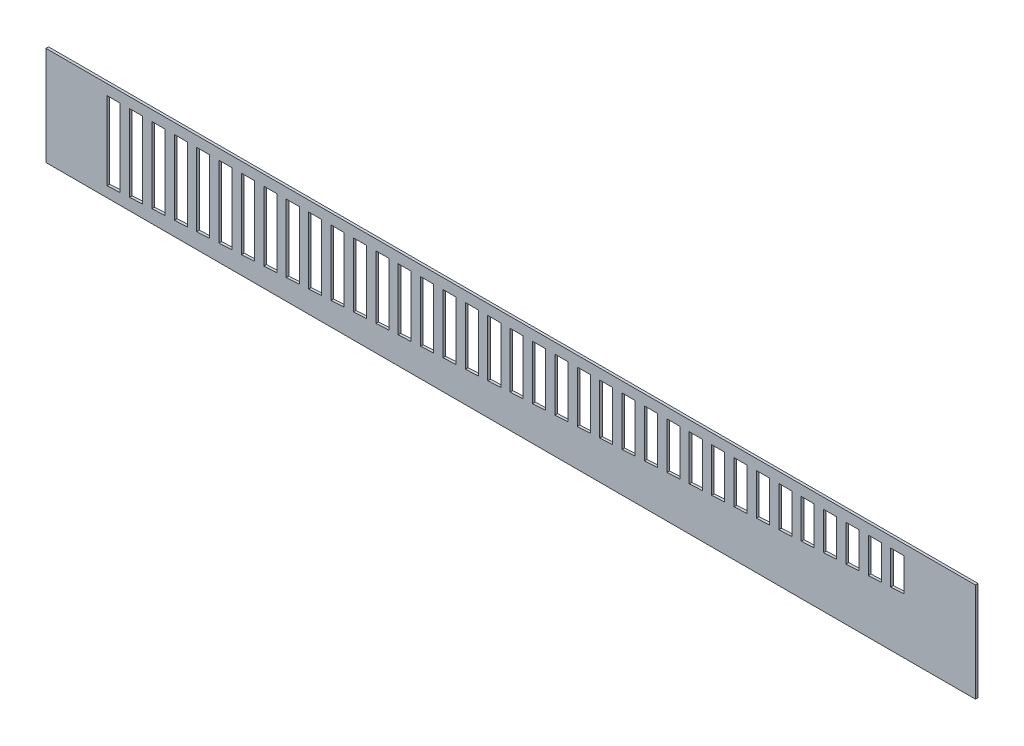
from build123d import *

# Parameters (mm, degrees)
SKETCH1_W           = 178.5
SKETCH1_H           = 19
BOSS_EXTRUDE1_DEPTH = 0.5
CUT_EXTRUDE1_DEPTH  = 147.56


with BuildPart() as part:
    # Sketch1 → Boss-Extrude1 (new body)
    with BuildSketch(Plane.XY):
        Rectangle(SKETCH1_W, SKETCH1_H)
    extrude(amount=BOSS_EXTRUDE1_DEPTH)

    # Sketch2 → Cut-Extrude1 (cut)
    with BuildSketch(Plane.XY.offset(0.5)):
        Polygon((-77.51, 7.5), (-75.01, 7.5), (-75.01, -7.358477447), (-77.51, -7.5), align=None)
        Polygon((-70.71, 7.5), (-70.71, -7.115058656), (-73.21, -7.256581209), (-73.21, 7.5), align=None)
        Polygon((-66.41, 7.5), (-66.41, -6.871639865), (-68.91, -7.013162418), (-68.91, 7.5), align=None)
        Polygon((-62.11, 7.5), (-62.11, -6.628221074), (-64.61, -6.769743627), (-64.61, 7.5), align=None)
        Polygon((-57.81, 7.5), (-57.81, -6.384802283), (-60.31, -6.526324836), (-60.31, 7.5), align=None)
        Polygon((-53.51, 7.5), (-53.51, -6.141383492), (-56.01, -6.282906045), (-56.01, 7.5), align=None)
        Polygon((-49.21, 7.5), (-49.21, -5.897964701), (-51.71, -6.039487254), (-51.71, 7.5), align=None)
        Polygon((-44.91, 7.5), (-44.91, -5.65454591), (-47.41, -5.796068463), (-47.41, 7.5), align=None)
        Polygon((-40.61, 7.5), (-40.61, -5.411127119), (-43.11, -5.552649672), (-43.11, 7.5), align=None)
        Polygon((-36.31, 7.5), (-36.31, -5.167708328), (-38.81, -5.309230881), (-38.81, 7.5), align=None)
        Polygon((-32.01, 7.5), (-32.01, -4.924289537), (-34.51, -5.06581209), (-34.51, 7.5), align=None)
        Polygon((-27.71, 7.5), (-27.71, -4.680870746), (-30.21, -4.822393299), (-30.21, 7.5), align=None)
        Polygon((-23.41, 7.5), (-23.41, -4.437451955), (-25.91, -4.578974508), (-25.91, 7.5), align=None)
        Polygon((-19.11, 7.5), (-19.11, -4.194033164), (-21.61, -4.335555717), (-21.61, 7.5), align=None)
        Polygon((-14.81, 7.5), (-14.81, -3.950614373), (-17.31, -4.092136926), (-17.31, 7.5), align=None)
        Polygon((-10.51, 7.5), (-10.51, -3.707195582), (-13.01, -3.848718135), (-13.01, 7.5), align=None)
        Polygon((-6.21, 7.5), (-6.21, -3.463776791), (-8.71, -3.605299344), (-8.71, 7.5), align=None)
        Polygon((-1.91, 7.5), (-1.91, -3.220358), (-4.41, -3.361880553), (-4.41, 7.5), align=None)
        Polygon((2.39, 7.5), (2.39, -2.976939209), (-0.11, -3.118461762), (-0.11, 7.5), align=None)
        Polygon((6.69, 7.5), (6.69, -2.733520418), (4.19, -2.875042971), (4.19, 7.5), align=None)
        Polygon((10.99, 7.5), (10.99, -2.490101627), (8.49, -2.63162418), (8.49, 7.5), align=None)
        Polygon((15.29, 7.5), (15.29, -2.246682836), (12.79, -2.388205389), (12.79, 7.5), align=None)
        Polygon((19.59, 7.5), (19.59, -2.003264045), (17.09, -2.144786598), (17.09, 7.5), align=None)
        Polygon((23.89, 7.5), (23.89, -1.759845254), (21.39, -1.901367807), (21.39, 7.5), align=None)
        Polygon((28.19, 7.5), (28.19, -1.516426463), (25.69, -1.657949016), (25.69, 7.5), align=None)
        Polygon((32.49, 7.5), (32.49, -1.273007672), (29.99, -1.414530225), (29.99, 7.5), align=None)
        Polygon((36.79, 7.5), (36.79, -1.029588881), (34.29, -1.171111434), (34.29, 7.5), align=None)
        Polygon((41.09, 7.5), (41.09, -0.78617009), (38.59, -0.927692643), (38.59, 7.5), align=None)
        Polygon((45.39, 7.5), (45.39, -0.542751299), (42.89, -0.684273852), (42.89, 7.5), align=None)
        Polygon((49.69, 7.5), (49.69, -0.299332508), (47.19, -0.440855061), (47.19, 7.5), align=None)
        Polygon((53.99, 7.5), (53.99, -0.055913717), (51.49, -0.19743627), (51.49, 7.5), align=None)
        Polygon((58.29, 7.5), (58.29, 0.187505074), (55.79, 0.045982521), (55.79, 7.5), align=None)
        Polygon((62.59, 7.5), (62.59, 0.430923865), (60.09, 0.289401312), (60.09, 7.5), align=None)
        Polygon((66.89, 7.5), (66.89, 0.674342656), (64.39, 0.532820103), (64.39, 7.5), align=None)
        Polygon((71.19, 7.5), (71.19, 0.917761447), (68.69, 0.776238894), (68.69, 7.5), align=None)
        Polygon((75.49, 7.5), (75.49, 1.161180238), (72.99, 1.019657685), (72.99, 7.5), align=None)
    extrude(amount=-CUT_EXTRUDE1_DEPTH, mode=Mode.SUBTRACT)


solid = part.part
